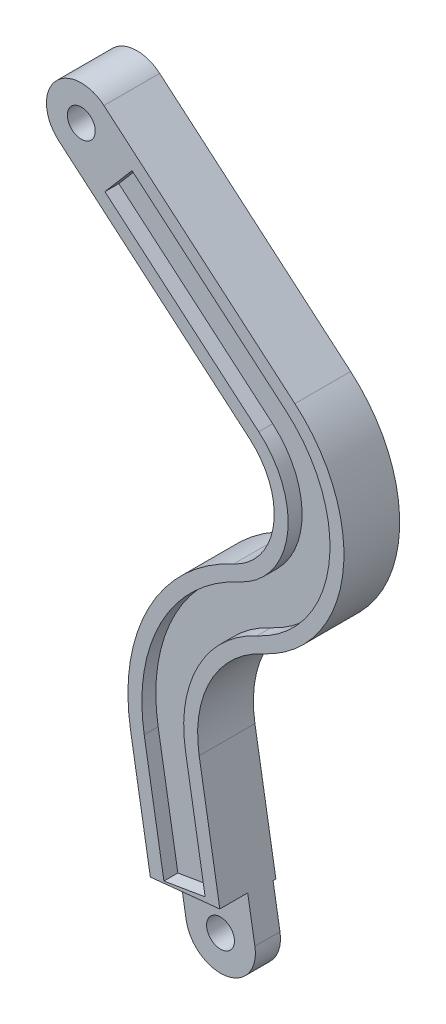
from build123d import *

# Parameters (mm, degrees)
BOSS_EXTRUDE1_DEPTH = 10
BOSS_EXTRUDE2_START = -20
BOSS_EXTRUDE2_DEPTH = 20
BOSS_EXTRUDE3_DEPTH = 10
SKETCH6_W           = 47.967212756
SKETCH6_H           = 31.917124467
CUT_EXTRUDE1_DEPTH  = 1
CUT_EXTRUDE2_DEPTH  = 10


with BuildPart() as part:
    # Sketch2 → Boss-Extrude1 (new body)
    with BuildSketch(Plane.XY):
        with BuildLine():
            Line((567.746058529, 114.079925051), (622.940708708, 67.071408889))
            ThreePointArc((622.940708708, 67.071408889), (633.205576943, 40.118894124), (616.005456238, 16.96805354))
            ThreePointArc((616.005456238, 16.96805354), (587.978717163, -9.525484834), (581.845382902, -47.601565115))
            Line((581.845382902, -47.601565115), (588.918006227, -89.508939159))
            Line((588.918006227, -89.508939159), (603.708844125, -87.012719162))
            Line((603.708844125, -87.012719162), (596.6362208, -45.105345118))
            ThreePointArc((596.6362208, -45.105345118), (601.237559856, -16.539976295), (622.263729898, 3.335958661))
            ThreePointArc((622.263729898, 3.335958661), (648.063910956, 38.062219537), (632.666608603, 78.490991685))
            Line((632.666608603, 78.490991685), (577.471958425, 125.499507846))
            Line((577.471958425, 125.499507846), (567.746058529, 114.079925051))
        make_face()
    extrude(amount=-BOSS_EXTRUDE1_DEPTH)

    # Sketch3 → Boss-Extrude2 (add)
    with BuildSketch(Plane.XY.offset(5).offset(BOSS_EXTRUDE2_START)):
        with BuildLine():
            Line((608.971952758, -88.152757549), (601.566500099, -44.273271785))
            ThreePointArc((601.566500099, -44.273271785), (605.657174086, -18.878140116), (624.349821118, -1.208072965))
            ThreePointArc((624.349821118, -1.208072965), (653.01668896, 37.376661342), (635.908575235, 82.297519283))
            Line((635.908575235, 82.297519283), (567.391078462, 140.652918656))
            ThreePointArc((567.391078462, 140.652918656), (549.769842886, 139.241516239), (551.181245303, 121.620280664))
            Line((551.181245303, 121.620280664), (619.698742076, 63.264881291))
            ThreePointArc((619.698742076, 63.264881291), (628.252798938, 40.80445232), (613.919365017, 21.512085166))
            ThreePointArc((613.919365017, 21.512085166), (583.559102933, -7.187321014), (576.915103602, -48.433638447))
            Line((576.915103602, -48.433638447), (584.320556261, -92.313124211))
            Line((584.320556261, -92.313124211), (608.971952758, -88.152757549))
        make_face()
        with BuildLine():
            Line((577.471958425, 125.499507846), (567.746058529, 114.079925051))
            Line((567.746058529, 114.079925051), (622.940708708, 67.071408889))
            ThreePointArc((622.940708708, 67.071408889), (633.205576943, 40.118894124), (616.005456238, 16.96805354))
            ThreePointArc((616.005456238, 16.96805354), (587.978717163, -9.525484834), (581.845382902, -47.601565115))
            Line((581.845382902, -47.601565115), (588.918006227, -89.508939159))
            Line((588.918006227, -89.508939159), (603.708844125, -87.012719162))
            Line((603.708844125, -87.012719162), (596.6362208, -45.105345118))
            ThreePointArc((596.6362208, -45.105345118), (601.237559856, -16.539976295), (622.263729898, 3.335958661))
            ThreePointArc((622.263729898, 3.335958661), (648.063910956, 38.062219537), (632.666608603, 78.490991685))
            Line((632.666608603, 78.490991685), (577.471958425, 125.499507846))
        make_face(mode=Mode.SUBTRACT)
        with BuildLine():
            ThreePointArc((558.45408855, 136.066878959), (554.355882583, 130.304526327), (560.118235215, 126.20632036))
            ThreePointArc((560.118235215, 126.20632036), (564.216441182, 131.968672992), (558.45408855, 136.066878959))
        make_face(mode=Mode.SUBTRACT)
    extrude(amount=BOSS_EXTRUDE2_DEPTH)

    # Sketch4 → Boss-Extrude3 (add)
    with BuildSketch(Plane.XY.offset(-5)):
        with BuildLine():
            Line((608.696660412, -86.521569404), (584.013862627, -90.495874195))
            Line((584.013862627, -90.495874195), (586.899983592, -107.596990039))
            ThreePointArc((586.899983592, -107.596990039), (601.305865171, -117.842504957), (611.551380088, -103.436623377))
            Line((611.551380088, -103.436623377), (608.696660412, -86.521569404))
        make_face()
        with BuildLine():
            ThreePointArc((598.393608507, -100.586527409), (594.295402541, -106.348880041), (600.057755172, -110.447086008))
            ThreePointArc((600.057755172, -110.447086008), (604.155961139, -104.684733376), (598.393608507, -100.586527409))
        make_face(mode=Mode.SUBTRACT)
    extrude(amount=-BOSS_EXTRUDE3_DEPTH)

    # Sketch6 → Cut-Extrude1 (cut)
    with BuildSketch(Plane(origin=(0, 0, -15), x_dir=(-1, 0, 0), z_dir=(0, 0, -1))):
        with Locations((-595.88807181, -104.755141446)):
            Rectangle(SKETCH6_W, SKETCH6_H)
    extrude(amount=-CUT_EXTRUDE1_DEPTH, mode=Mode.SUBTRACT)

    # Sketch7 → Cut-Extrude2 (cut)
    with BuildSketch(Plane.XY.offset(5)):
        Polygon((608.971952758, -88.152757549), (584.051383166, -90.718194429), (584.320556261, -92.313124211), align=None)
    extrude(amount=-CUT_EXTRUDE2_DEPTH, mode=Mode.SUBTRACT)


solid = part.part
